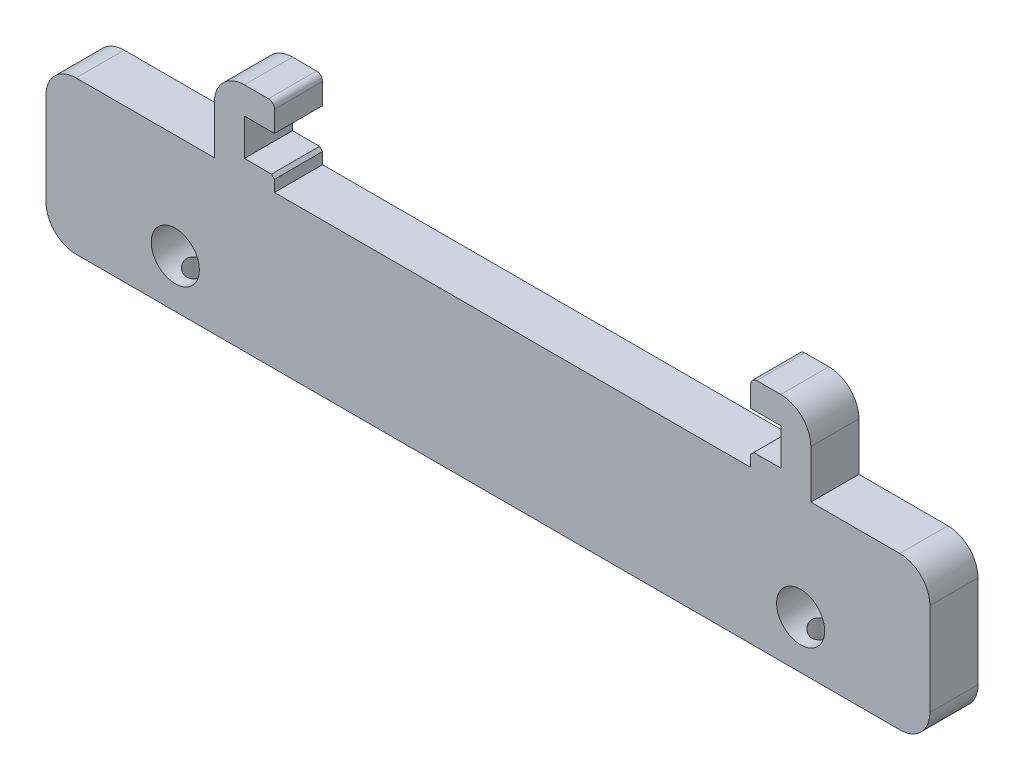
from build123d import *

# Parameters (mm, degrees)
SKETCH1_W                      = 147
SKETCH1_H                      = 25.4
BOSS_EXTRUDE1_DEPTH            = 8
SKETCH2_W                      = 5
SKETCH2_H                      = 8
BOSS_EXTRUDE2_DEPTH            = 10
SKETCH3_W                      = 8
SKETCH3_H                      = 1.5
BOSS_EXTRUDE3_DEPTH            = 5
SKETCH4_W                      = 5
SKETCH4_H                      = 8
BOSS_EXTRUDE4_DEPTH            = 2.4
SKETCH7_R                      = 4
CUT_EXTRUDE1_DEPTH             = 150.392637034
SKETCH8_W                      = 10
SKETCH8_H                      = 8
BOSS_EXTRUDE5_DEPTH            = 3
FILLET1_R                      = 5
CHAMFER1_SIZE                  = 0.5
F_4_2_4_2_DIAMETER_HOLE1_D     = 4.2
F_4_2_4_2_DIAMETER_HOLE1_DEPTH = 9.5
F_4_2_4_2_DIAMETER_HOLE1_TIP   = 1.2618073
FILLET2_R                      = 5
FILLET3_R                      = 1


with BuildPart() as part:
    # Sketch1 → Boss-Extrude1 (new body)
    with BuildSketch(Plane.XY):
        with Locations((73.5, -12.7)):
            Rectangle(SKETCH1_W, SKETCH1_H)
    extrude(amount=BOSS_EXTRUDE1_DEPTH)

    # Sketch2 → Boss-Extrude2 (add)
    with BuildSketch(Plane(origin=(0, 0, 0), x_dir=(1, 0, 0), z_dir=(0, 1, 0))):
        with Locations((124.7, -4)):
            Rectangle(SKETCH2_W, SKETCH2_H)
        with Locations((30.5, -4)):
            Rectangle(SKETCH2_W, SKETCH2_H)
    extrude(amount=BOSS_EXTRUDE2_DEPTH)

    # Sketch3 → Boss-Extrude3 (add)
    with BuildSketch(Plane(origin=(33, 0, 0), x_dir=(0, 0, -1), z_dir=(1, 0, 0))):
        with Locations((-4, 9.25)):
            Rectangle(SKETCH3_W, SKETCH3_H)
    boss_extrude3 = extrude(amount=BOSS_EXTRUDE3_DEPTH)

    # Mirror1: Boss-Extrude3 across plane
    add(boss_extrude3.mirror(Plane(origin=(77.6, 0, 0), x_dir=(0, 0, 1), z_dir=(1, 0, 0))))

    # Sketch4 → Boss-Extrude4 (add)
    with BuildSketch(Plane(origin=(0, 0, 0), x_dir=(1, 0, 0), z_dir=(0, 1, 0))):
        with Locations((35.5, -4)):
            Rectangle(SKETCH4_W, SKETCH4_H)
        with Locations((119.7, -4)):
            Rectangle(SKETCH4_W, SKETCH4_H)
    extrude(amount=BOSS_EXTRUDE4_DEPTH)

    # Sketch7 → Cut-Extrude1 (cut, through all)
    with BuildSketch(Plane.XY.offset(8)):
        with Locations((21.5, -17.4)):
            Circle(SKETCH7_R)
        with Locations((125.5, -17.4)):
            Circle(SKETCH7_R)
    extrude(amount=-CUT_EXTRUDE1_DEPTH, mode=Mode.SUBTRACT)

    # Sketch8 → Boss-Extrude5 (add)
    with BuildSketch(Plane(origin=(0, 10, 0), x_dir=(1, 0, 0), z_dir=(0, 1, 0))):
        with Locations((33, -4)):
            Rectangle(SKETCH8_W, SKETCH8_H)
        with Locations((122.2, -4)):
            Rectangle(SKETCH8_W, SKETCH8_H)
    extrude(amount=BOSS_EXTRUDE5_DEPTH)

    # Fillet1
    fillet1_edges = [part.edges().sort_by_distance(p)[0] for p in [
        (28, 13, 4),
        (127.2, 13, 4),
        (0, 0, 4),
        (147, 0, 4),
    ]]
    fillet(fillet1_edges, radius=FILLET1_R)

    # Chamfer1
    chamfer1_edges = [part.edges().sort_by_distance(p)[0] for p in [
        (38, 2.4, 4),
        (117.2, 2.4, 4),
    ]]
    chamfer(chamfer1_edges, length=CHAMFER1_SIZE)

    # Ø4.2 (4.2) Diameter Hole1
    with Locations(Plane.XZ.offset(25.4)):
        with Locations((21.5, 4), (125.5, 4)):
            Hole(F_4_2_4_2_DIAMETER_HOLE1_D / 2, depth=F_4_2_4_2_DIAMETER_HOLE1_DEPTH)
            with Locations((0, 0, -(F_4_2_4_2_DIAMETER_HOLE1_DEPTH + F_4_2_4_2_DIAMETER_HOLE1_TIP / 2))):  # 118° drill point
                Cone(0, F_4_2_4_2_DIAMETER_HOLE1_D / 2, F_4_2_4_2_DIAMETER_HOLE1_TIP, mode=Mode.SUBTRACT)

    # Fillet2
    fillet2_edges = [part.edges().sort_by_distance(p)[0] for p in [
        (147, -25.4, 4),
        (0, -25.4, 4),
    ]]
    fillet(fillet2_edges, radius=FILLET2_R)

    # Fillet3
    fillet3_edges = [part.edges().sort_by_distance(p)[0] for p in [
        (38, 13, 4),
        (117.2, 13, 4),
    ]]
    fillet(fillet3_edges, radius=FILLET3_R)


solid = part.part
